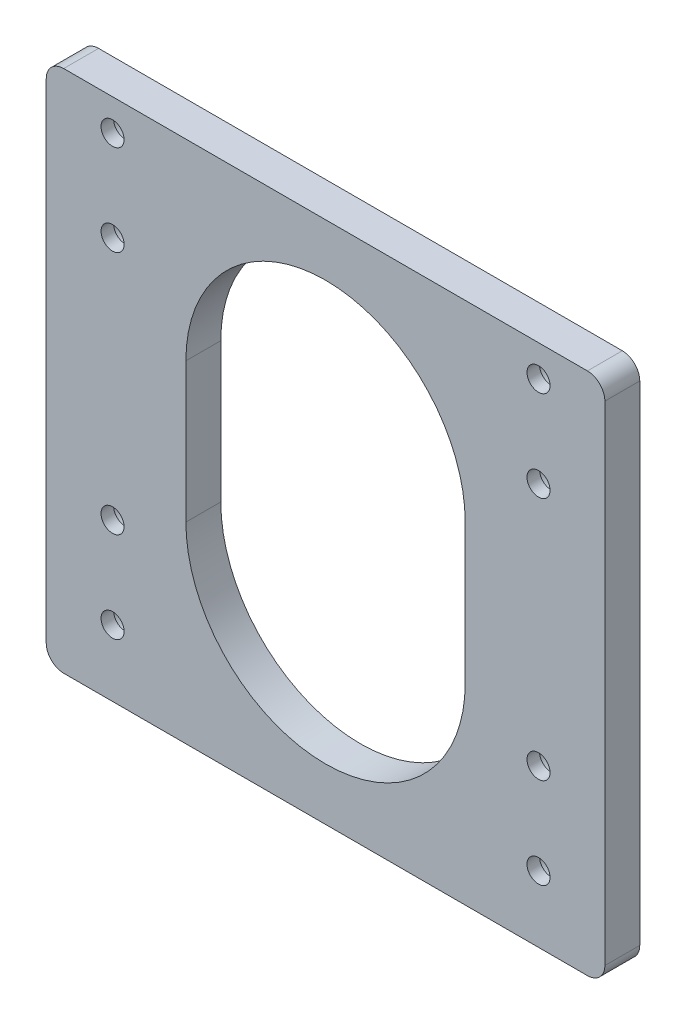
SolidWorks part; units mm, degrees
material "SUS304"
ref_plane "前视基准面" through (0, 0, 0) normal (0, 0, 1) x (1, 0, 0)
ref_plane "上视基准面" through (0, 0, 0) normal (0, 1, 0) x (1, 0, 0)
ref_plane "右视基准面" through (0, 0, 0) normal (1, 0, 0) x (0, 0, -1)
sketch "草图1" plane through (0, 0, 0) normal (0, 0, 1) x (1, 0, 0)
  line L1 (28883.6203, 93.5657) -> (29043.6203, 93.5657)
  line L2 (28883.6203, 93.5657) -> (28883.6203, -56.4343)
  line L3 (28883.6203, -56.4343) -> (29043.6203, -56.4343)
  line L4 (29043.6203, 93.5657) -> (29043.6203, -56.4343)
  dimension "D1" = 160
  dimension "D2" = 150
extrude "凸台-拉伸1" add sketch "草图1" along normal blind 10
fillet "圆角1" radius 5 4 edges at (28883.6203, 93.5657, 5) (29043.6203, -56.4343, 5) (28883.6203, -56.4343, 5) (29043.6203, 93.5657, 5)
hole_wizard "M6 六角凹头螺钉的柱形沉头孔1" positions "草图2" profile "草图3" counterbore size "M6" standard "ISO"
sketch "草图2" plane through (0, 0, 0) normal (0, 0, -1) x (-1, 0, 0)
  line L0 (-28963.6203, -56.4343) -> (-28963.6203, -79.7742) construction
  line L1 (-28888.6203, -56.4343) -> (-29038.6203, -56.4343) construction
  point P3 (-29024.6203, 84.5657)
  point P5 (-29024.6203, 58.5657)
  point P7 (-29024.6203, -11.4343)
  point P9 (-29024.6203, -37.4343)
  point P17 (-28902.6203, -37.4343)
  point P18 (-28902.6203, -11.4343)
  point P19 (-28902.6203, 58.5657)
  point P20 (-28902.6203, 84.5657)
sketch "草图3" plane through (29024.6203, 84.5657, 0) normal (1, 0, 0) x (0, 1, 0)
  line L0 (0, 0) -> (0, 13.4828)
  line L1 (0, 13.4828) -> (3.3, 11.5)
  line L2 (3.3, 11.5) -> (3.3, 6.4)
  line L3 (3.3, 6.4) -> (5.5, 6.4)
  line L4 (5.5, 6.4) -> (5.5, 0)
  line L5 (5.5, 0) -> (0, 0)
  line L10 (0, 13.4828) -> (-3.3, 11.5) construction
  line L11 (0, -6.35) -> (0, 107.95) construction
  dimension "孔直径" = 6.6
  dimension "孔深度" = 11.5
  dimension "柱形沉头孔直径" = 11
  dimension "柱形沉头孔深度" = 6.4
  dimension "导头角度" = 118
sketch "草图4" plane through (0, 0, 10) normal (0, 0, 1) x (1, 0, 0)
  line L0 (28963.6203, -1.4343) -> (28963.6203, 38.5657) construction
  line L1 (28923.6203, -1.4343) -> (28923.6203, 38.5657)
  line L2 (29003.6203, -1.4343) -> (29003.6203, 38.5657)
  line L3 (28963.6203, 18.5657) -> (28963.6203, -56.4343) construction
  line L4 (28888.6203, -56.4343) -> (29038.6203, -56.4343) construction
  line L5 (28963.6203, 18.5657) -> (28883.6203, 18.5657) construction
  line L6 (28883.6203, 88.5657) -> (28883.6203, -51.4343) construction
  arc A0 (28923.6203, -1.4343) -> (29003.6203, -1.4343) centre (28963.6203, -1.4343) ccw
  arc A1 (29003.6203, 38.5657) -> (28923.6203, 38.5657) centre (28963.6203, 38.5657) ccw
  point P2 (28963.6203, 18.5657)
  dimension "D2" = 40
  dimension "D1" = 40
extrude "切除-拉伸1" cut sketch "草图4" against normal blind 10
